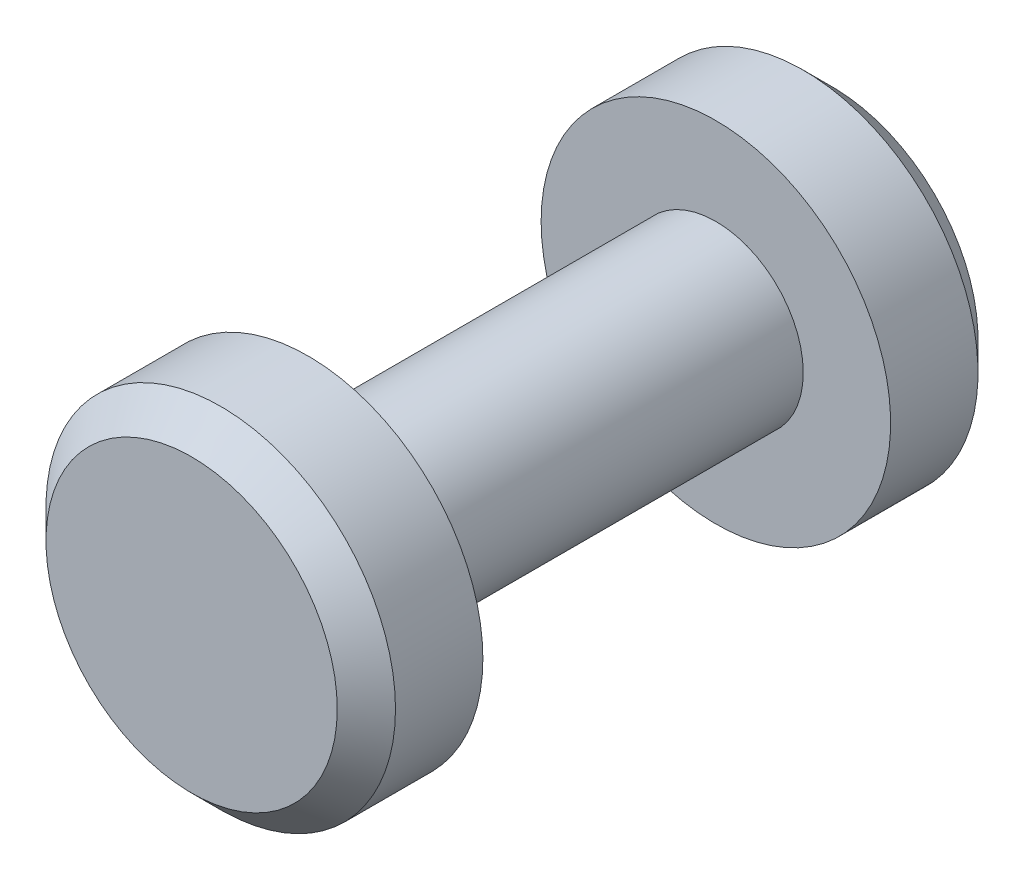
from build123d import *

# Parameters (mm, degrees)
SKETCH_1_R      = 3
EXTRUDE_1_DEPTH = 14
SKETCH_2_R      = 6
EXTRUDE_2_DEPTH = 4
CHAMFER_1_SIZE  = 1
EXTRUDE_START   = 4
SKETCH_3_R      = 6
EXTRUDE_3_DEPTH = 4
CHAMFER_2_SIZE  = 1


with BuildPart() as part:
    # 草图1 → 凸台-拉伸1 (new body)
    with BuildSketch(Plane.XY):
        Circle(SKETCH_1_R)
    extrude(amount=EXTRUDE_1_DEPTH)

    # 草图2 → 凸台-拉伸2 (add)
    with BuildSketch(Plane.XY.offset(14)):
        Circle(SKETCH_2_R)
    extrude(amount=EXTRUDE_2_DEPTH)

    # 倒角1
    chamfer_1_edges = [part.edges().sort_by_distance(p)[0] for p in [
        (-6, 0, 18),
    ]]
    chamfer(chamfer_1_edges, length=CHAMFER_1_SIZE)

    # 草图3 → 凸台-拉伸3 (add)
    with BuildSketch(Plane(origin=(0, 0, 0), x_dir=(-1, 0, 0), z_dir=(0, 0, -1)).offset(EXTRUDE_START)):
        with Locations(Location((0, 0, 0), (0, 0, 180))):
            Circle(SKETCH_3_R)
    extrude(amount=-EXTRUDE_3_DEPTH)

    # 倒角2
    chamfer_2_edges = [part.edges().sort_by_distance(p)[0] for p in [
        (-6, 0, -4),
    ]]
    chamfer(chamfer_2_edges, length=CHAMFER_2_SIZE)


solid = part.part
